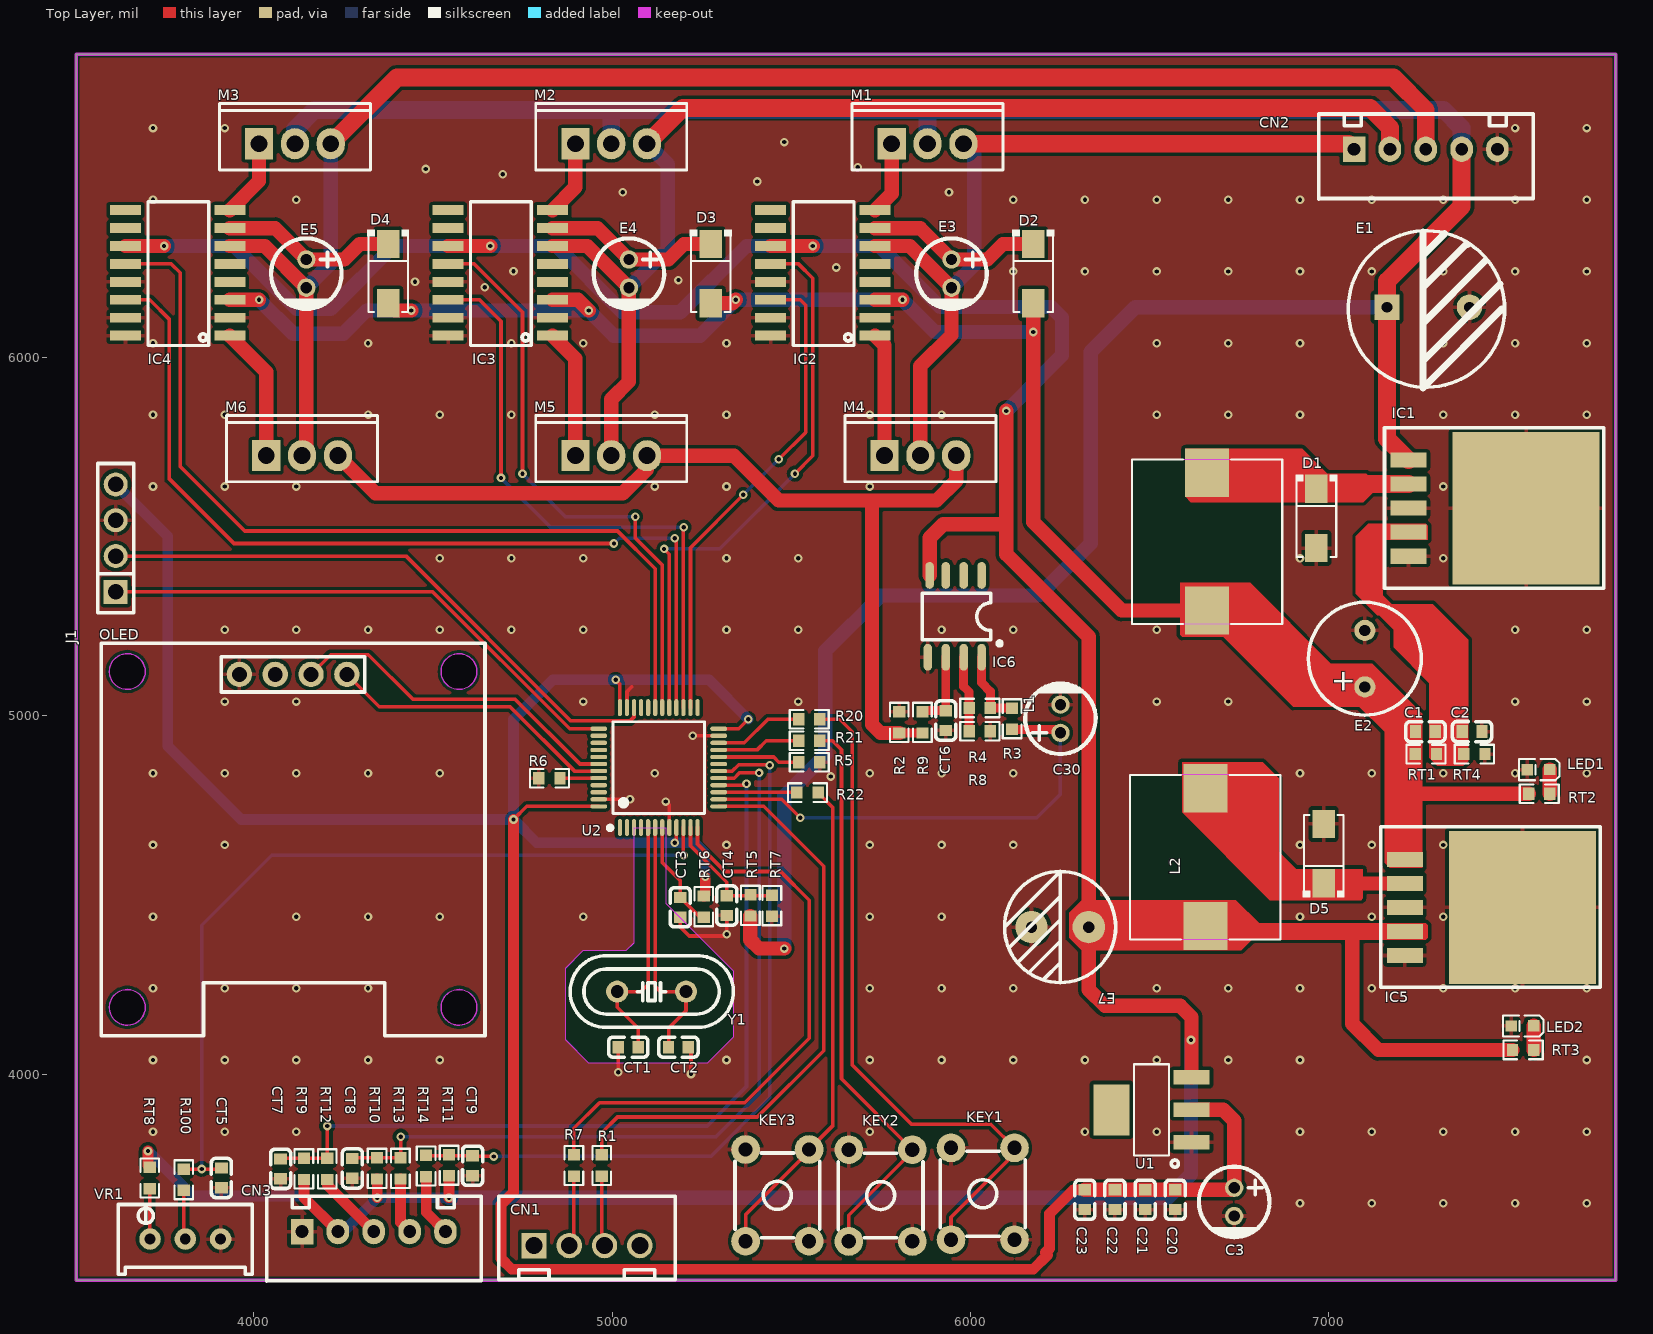
[diagram p0: Top Layer view]
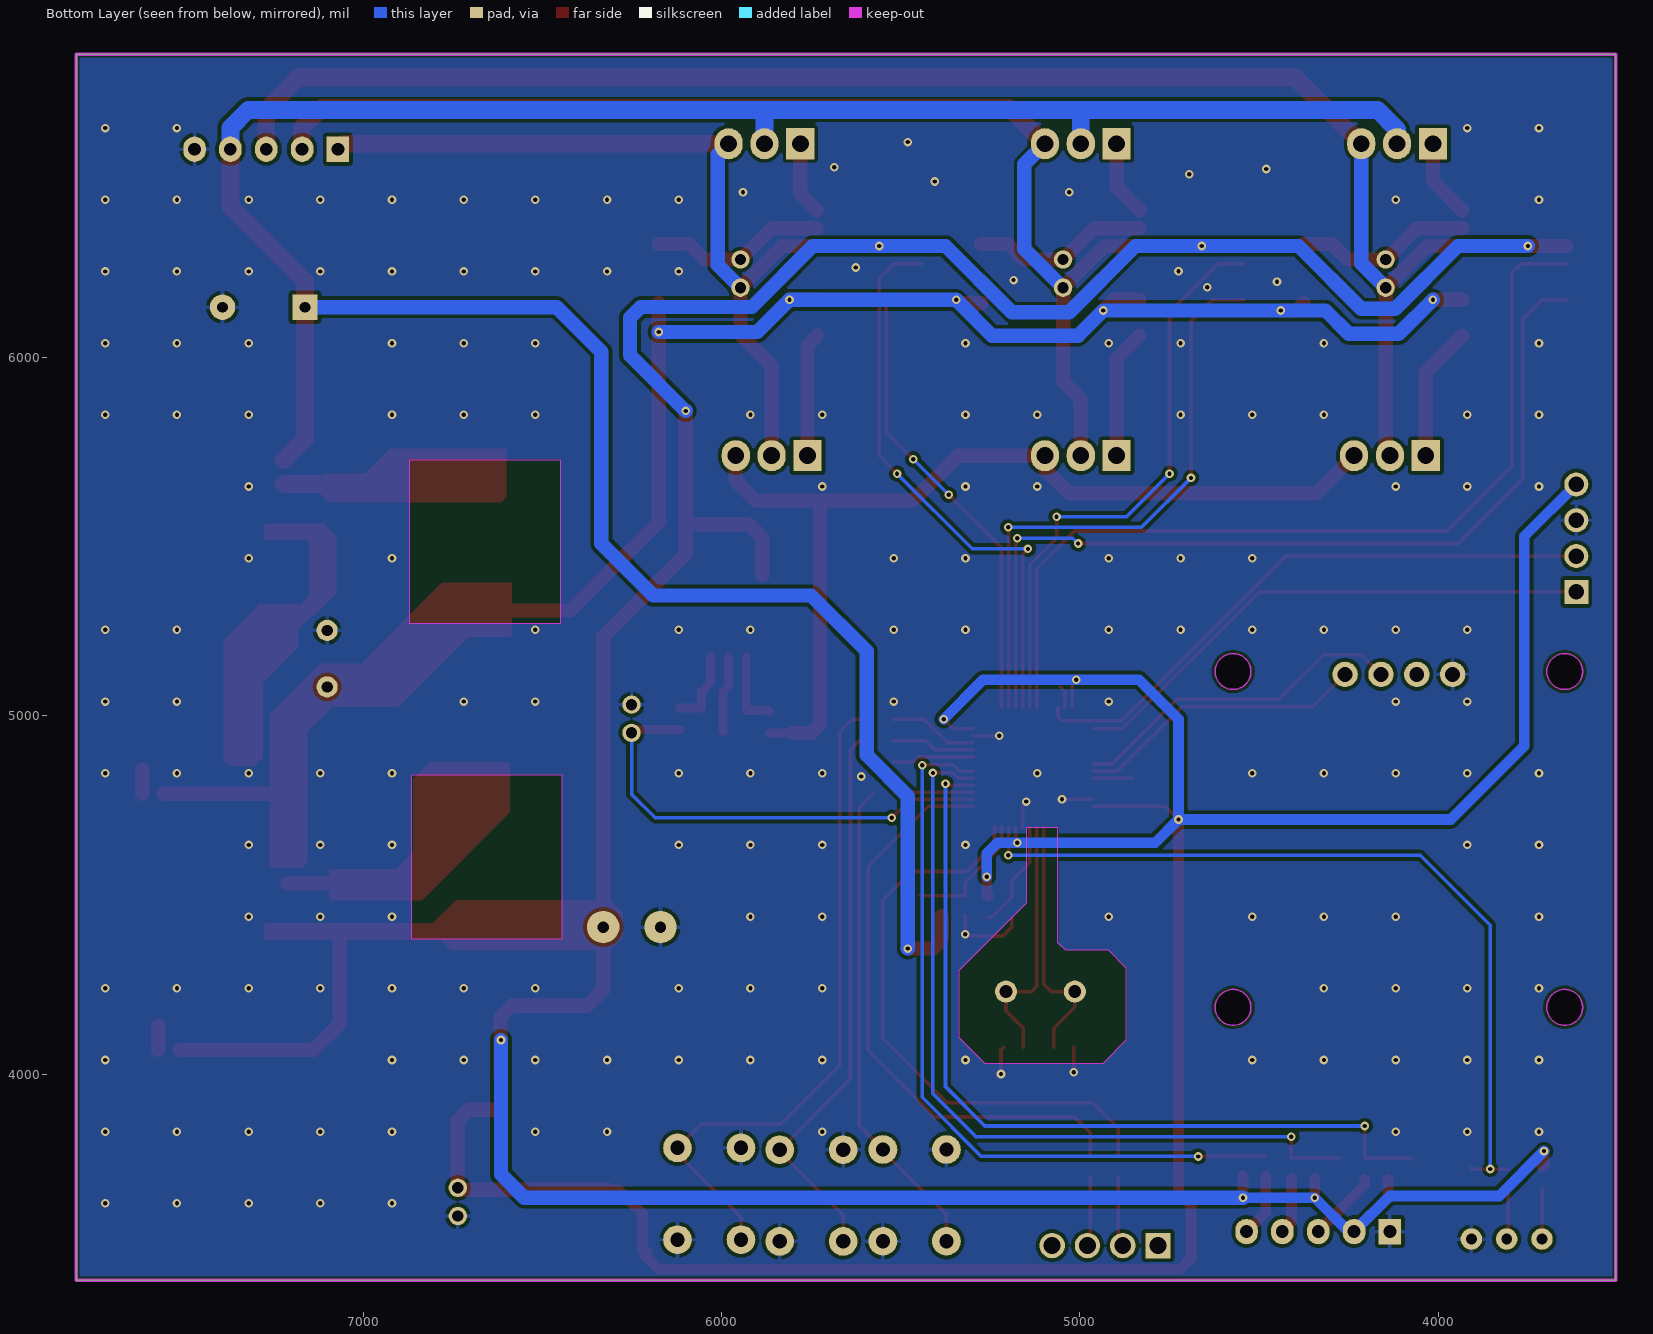
[diagram p1: Bottom Layer view, seen from below]
# Altium PCB MISC58867.pcbdoc
Units mil, origin at the board's own origin, x right, y up, seen from the top; angles counter-clockwise.
Board outline 4295 x 3420 mil, 2 copper layers (Top Layer, Bottom Layer), stack 62.206 mil thick; 83 components, 79 nets, 295 pads, 220 vias.

## Layer stack, top to bottom
Top Solder Mask Layer: solder mask 0.394, Dk 3.3
Top Layer: signal copper 1.379
Dielectric1: surface 59.449, FR4, Dk 4.5
Bottom Layer: signal copper 1.378
Bottom Solder Mask Layer: solder mask 0.394, Dk 3.3

## Board outline
3505,6845 3505,3425 7800,3425 7800,6845

## Design rules (kind name [scope] priority, off if disabled: settings)
BoardOutlineClearance copperThickness2oz_1 [All] p2 off: genericclearance=7.99 ignorepadtopadclearanceinfootprint=FALSE except(0: Arc-SplitContinuation Track-SplitContinuation SMDPad-SplitContinuation THPad-SplitContinuation Via-SplitContinuation Fill-SplitContinuation Region-SplitContinuation Poly-SplitContinuation Text-SplitContinuation Hole-SplitContinuation; 5.98: Arc-CutoutEdge SMDPad-CutoutEdge THPad-CutoutEdge Via-CutoutEdge Fill-CutoutEdge Region-CutoutEdge Text-CutoutEdge; 6.93: Hole-OutlineEdge Hole-CutoutEdge; 10: Poly-OutlineEdge Poly-CutoutEdge; 11.81: Arc-OutlineEdge Track-OutlineEdge SMDPad-OutlineEdge THPad-OutlineEdge Via-OutlineEdge Fill-OutlineEdge Region-OutlineEdge Text-OutlineEdge Track-CutoutEdge)
BoardOutlineClearance copperThickness1oz_1 [All] p4: genericclearance=4.02 ignorepadtopadclearanceinfootprint=FALSE except(0: Arc-SplitContinuation Track-SplitContinuation SMDPad-SplitContinuation THPad-SplitContinuation Via-SplitContinuation Fill-SplitContinuation Region-SplitContinuation Poly-SplitContinuation Text-SplitContinuation Hole-SplitContinuation; 6: SMDPad-CutoutEdge THPad-CutoutEdge Via-CutoutEdge Fill-CutoutEdge Region-CutoutEdge Text-CutoutEdge; 6.93: Hole-OutlineEdge Hole-CutoutEdge; 10: Poly-OutlineEdge Poly-CutoutEdge; 11.8: Arc-OutlineEdge Track-OutlineEdge SMDPad-OutlineEdge THPad-OutlineEdge Via-OutlineEdge Fill-OutlineEdge Region-OutlineEdge Text-OutlineEdge; 11.81: Arc-CutoutEdge Track-CutoutEdge)
Clearance copperThickness2oz [All] p1 off: gap=7.99 ignorepadtopadclearanceinfootprint=FALSE except(5.98: SMDPad-Track SMDPad-SMDPad THPad-Track SMDPad-THPad THPad-THPad Track-Via SMDPad-Via THPad-Via Via-Via Fill-Track Region-Track Fill-SMDPad Region-SMDPad Fill-THPad Region-THPad Fill-Via Region-Via Fill-Fill Fill-Region Region-Region Arc-Track Arc-SMDPad Arc-THPad Arc-Via Fill-Arc Region-Arc Arc-Arc Text-Track SMDPad-Text Text-THPad Text-Via Fill-Text Region-Text Arc-Text Text-Text; 6.93: Hole-Track Hole-SMDPad Hole-THPad Hole-Via Fill-Hole Region-Hole Hole-Arc Hole-Text; 10: Poly-Track Poly-SMDPad Poly-THPad Poly-Via Poly-Fill Poly-Region Poly-Poly Poly-Arc Poly-Text Poly-Hole)
Clearance copperThickness1oz [All] p3: gap=4.02 ignorepadtopadclearanceinfootprint=FALSE except(5.98: SMDPad-Track SMDPad-SMDPad THPad-Track SMDPad-THPad THPad-THPad Track-Via SMDPad-Via THPad-Via Via-Via Fill-Track Region-Track Fill-SMDPad Region-SMDPad Fill-THPad Region-THPad Fill-Via Region-Via Fill-Fill Fill-Region Region-Region; 6: Arc-Track Arc-SMDPad Arc-THPad Arc-Via Fill-Arc Region-Arc Arc-Arc Text-Track SMDPad-Text Text-THPad Text-Via Fill-Text Region-Text Arc-Text Text-Text; 6.93: Hole-Track Hole-SMDPad Hole-THPad Hole-Via Fill-Hole Region-Hole Hole-Arc Hole-Text; 10: Poly-Track Poly-SMDPad Poly-THPad Poly-Via Poly-Fill Poly-Region Poly-Poly Poly-Arc Poly-Text Poly-Hole)
Creepage creepage [All] p1: checkdistance=0 ignoreinternallayers=TRUE applytopolygonpour=TRUE
DiffPairsRouting differentialPair [All] p1: maxlimit=6 minlimit=6 mostfreqgap=6 toplayer_minwidth=5 toplayer_prefwidth=10 toplayer_maxwidth=100 toplayer_mingap=6 toplayer_prefgap=6 toplayer_maxgap=6 bottomlayer_minwidth=5 bottomlayer_prefwidth=10 bottomlayer_maxwidth=100 bottomlayer_mingap=6 bottomlayer_prefgap=6 bottomlayer_maxgap=6 maxuncoupledlength=10
HoleToHoleClearance otherClearance [All] p1: gap=11.81 allowstackedmicrovias=TRUE
Length netLength [All] p1: minlimit=0 maxlimit=0
MatchedLengths netLengthTolerance [All] p1: tolerance=1000
PasteMaskExpansion pasteMaskExpansion [All] p1: expansion=0
PlaneConnect innerPlane [All] p1: planeconnectstyle=Relief reliefexpansion=20 reliefentries=4 reliefconductorwidth=10 reliefairgap=10
PolygonConnect copperRegion [(InNet('GND'))] p1: connectstyle=Relief reliefconductorwidth=10 reliefentries=4 polygonreliefangle="90 Angle" airgapwidth=10 via.connectstyle=Relief via.reliefconductorwidth=10 via.reliefentries=4 via.polygonreliefangle="90 Angle" via.airgapwidth=10
RoutingVias viaSize [All] p1: holewidth=12.01 width=24.02 viastyle="Through Hole" minholewidth=11.81 minwidth=19.68 maxholewidth=248.03 maxwidth=393.7
SolderMaskExpansion solderMaskExpansion [IsVia] p1: expansion=-1000 istentingtop=TRUE
SolderMaskExpansion solderMaskExpansion [All] p2: expansion=2 istentingtop=FALSE
Width copperThickness2oz_2 [All] p1 off: maxlimit=100 minlimit=8 preferedwidth=10
Width copperThickness1oz_2 [All] p2: maxlimit=100 minlimit=5 preferedwidth=10

## Components (designator, comment, footprint, x,y, rotation, side; value= is the part's Value field where it differs from the comment)
C1 "104" C0603 7269.16,4955.29 r0 top
C2 "104" C0603 7399.04,4955.41 r0 top
C3 "16V/220uF" CAP-TH_BD5.0-P2.00-D0.8-FD-10UF50VC110GL 6735.51,3643.15 r270 top
C20 "104" C0603 6571.1,3649.32 r270 top
C21 "104" C0603 6486.97,3649.32 r270 top
C22 "104" C0603 6402.84,3649.32 r270 top
C23 "104" C0603 6318.71,3649.32 r270 top
C30 "106" CAP-TH_BD5.0-P2.00-D0.8-FD-10UF50VC110GL 6250.8,4991.13 r90 top
CN1 "CON4" CON4 4928.57,3546.8 r0 top
CN2 "CON5" CON5 7070,6580 r0 top
CN3 "CON5" CON5 4135.02,3560.37 r0 top
CT1 "30pf" C0603 5045,4075 r180 top
CT2 "30pf" C0603 5185,4075 r180 top
CT3 "105" C0603 5190,4465 r90 top
CT4 "104" C0603 5320,4470 r90 top
CT5 "104" C0603 3910,3710 r90 top
CT6 "104" C0603 5930.8,4986.13 r90 top
CT7 "104" C0603 4075.02,3735.37 r90 top
CT8 "104" C0603 4275.34,3736.44 r90 top
CT9 "104" C0603 4610.63,3744.01 r90 top
D1 "SS34/1N5822" SMA_L4.3-W2.5-LS5.0-RD 6965,5550 r270 top
D2 "M4" SMA_L4.3-W2.5-LS5.0-RD 6175,6232.84 r270 top
D3 "M4" SMA_L4.3-W2.5-LS5.0-RD 5275.07,6232.84 r270 top
D4 "M4" SMA_L4.3-W2.5-LS5.0-RD 4375.14,6232.84 r270 top
D5 "SS34/1N5822" SMA_L4.3-W2.5-LS5.0-RD 6985,4615 r90 top
E1 "50V/330uF" 50v/330uf 7271.97,6134.36 r0 top
E2 "50V/100uF" 50V/100UF 7100,5080 r90 top
E3 "10UF" CAP-TH_BD5.0-P2.00-D0.8-FD-10UF50VC110GL 5946.79,6233.03 r270 top
E4 "10UF" CAP-TH_BD5.0-P2.00-D0.8-FD-10UF50VC110GL 5046.86,6233.03 r270 top
E5 "10UF" CAP-TH_BD5.0-P2.00-D0.8-FD-10UF50VC110GL 4146.93,6233.03 r270 top
E7 "16V/220uF" 16V/220UF 6330,4410 r180 top
IC1 "LM2596S" LM2596S 7385.8,5578.56 r270 top
IC2 "IR2113S" SOP-16 5587.89,6235 r90 top
IC3 "IR2113S" SOP-16 4687.96,6235 r90 top
IC4 "IR2113S" SOP-16 3788.03,6235 r90 top
IC5 "LM2596S-5V" LM2596S 7375.8,4464.72 r270 top
IC6 "LM358" lm358 6030.8,5391.13 r180 top
J1 "CON4(NC)" HDR-TH_4P-P2.54-V-F 3615,5495 r90 top
KEY1 "" SW-PB1 6034.1,3665.9 r270 top
KEY2 "" SW-PB1 5749.1,3660.9 r270 top
KEY3 "" SW-PB1 5460.9,3661.42 r270 top
L1 "33UH/3A" IND-SMD_L11.5-W10.5_MWSA1004 6660,5485 r90 top
L2 "33UH/3A" IND-SMD_L11.5-W10.5_MWSA1004 6655,4605 r90 top
LED1 "REG" LED0603 7584.7,4849.32 r180 top
LED2 "REG" LED0603 7539.7,4134.32 r180 top
M1 "IR540" IR5401 5765,6620.31 r0 top
M2 "IR540" IR5401 4882.5,6620.31 r0 top
M3 "IR540" IR5401 4000,6620.31 r0 top
M4 "IR540" IR5401 5745,5750 r0 top
M5 "IR540" IR5401 4882.5,5750 r0 top
M6 "IR540" IR5401 4020,5750 r0 top
OLED "OLED" OLED 4110,5115 r0 top
R1 "100R" R0603 4970.98,3744.8 r90 top
R2 "0.22R" R0603 5800.8,4981.13 r90 top
R3 "1K" R0603 6115.8,4991.13 r90 top
R4 "10K" R0603 6025.8,5021.13 r0 top
R5 "4.7K" R0603 5550,4870 r180 top
R6 "4.7K" R0603 4825,4825 r0 top
R7 "100R" R0603 4893.28,3744.8 r90 top
R8 "1K" R0603 6025.8,4956.13 r0 top
R9 "1K" R0603 5865.8,4981.13 r90 top
R20 "10K" R0603 5550,4990 r0 top
R21 "10K" R0603 5550,4930 r0 top
R22 "10K" R0603 5545,4785 r0 top
R100 "1K" R0603 3805,3705 r270 top
RT1 "10K" R0603 7270.43,4892.62 r180 top
RT2 "1K" R0603 7586.66,4782 r180 top
RT3 "1K" R0603 7541.66,4067 r180 top
RT4 "1K" R0603 7405.43,4892.62 r180 top
RT5 "20K" R0603 5385.76,4470.48 r270 top
RT6 "10K" R0603 5255.65,4466.9 r90 top
RT7 "1K" R0603 5445.76,4469.52 r90 top
RT8 "5K" R0603 3710,3710 r90 top
RT9 "10K" R0603 4140.02,3735.37 r270 top
RT10 "10K" R0603 4344.26,3736.74 r270 top
RT11 "10K" R0603 4545.02,3745.37 r270 top
RT12 "220R" R0603 4205.02,3735.37 r270 top
RT13 "220R" R0603 4409.26,3736.74 r270 top
RT14 "220R" R0603 4481.13,3743.41 r270 top
U1 "1117-3.3V" 1117-3.3V 6505,3900 r180 top
U2 "STM32F103C8T6" STM32F103C8T6 5130,4855 r90 top
VR1 "10K" R_3296 3809.32,3544.52 r0 top
Y1 "8M" HC-49S_L11.5-W5.0-P4.88 5110,4230 r180 top

## Footprints (in the part's own frame and the unit in brackets; to place one, negate y for a bottom-side part, rotate by r counter-clockwise, add the part's x,y. Pads: shape width x height; smd on the part's side, far side on the other; paste and mask are expansions set on the pad)
16V/220UF [mm]
  round 2.3 hole 0.813 paste+0.051 mask+0.102: 1(0,0) 2(4.064,0)
  silkscreen extent -1.91,-3.94 5.97,3.94
50V/100UF [mm]
  round 1.5 hole 0.8: 1(0,0) 2(4,0)
  silkscreen extent -2,-4 6,4
50v/330uf [mil]
  rect 70.87x70.87 hole 30: 1(-110,5)
  round 70.87 hole 30: 2(120,5)
  silkscreen extent -218,-220 218,218
1117-3.3V [mm]
  rect 2.565x1.015 smd: 1(-2.832,2.3) 2(-2.832,0) 3(-2.832,-2.3)
  rect 2.565x3.6 smd: 4(2.832,0)
  silkscreen extent -1.9,-3.23 1.25,4.06
C0603 [mm]
  rect 0.8x0.9 smd: 1(-0.7,0) 2(0.7,0)
  silkscreen extent -1.39,-0.71 1.39,0.71
CAP-TH_BD5.0-P2.00-D0.8-FD-10UF50VC110GL [mm]
  round 1.3 hole 0.8: 1(-1,0) 2(1,0)
  silkscreen extent -2.5,-2.5 2.5,2.5
CON4 [mm]
  rect 1.8x1.8 hole 1.2: 1(-3.723,-0.648)
  round 1.8 hole 1.2: 2(-1.223,-0.648) 3(1.277,-0.648) 4(3.777,-0.648)
  silkscreen extent -6.22,-3.05 6.28,2.85
CON5 [mm]
  rect 1.6x1.8 hole 0.9: 1(0,0)
  oval 1.6x1.8 hole 0.9: 2(2.54,0) 3(5.08,0) 4(7.62,0) 5(10.16,0)
  silkscreen extent -2.5,-3.52 12.7,2.5
HC-49S_L11.5-W5.0-P4.88 [mm]
  round 1.56 hole 0.9: 1(-2.44,0) 2(2.44,0)
  silkscreen extent -5.8,-2.54 5.77,2.54
HDR-TH_4P-P2.54-V-F [mm]
  rect 1.7x1.7 hole 1.1: 1(-3.81,0)
  round 1.7 hole 1.1: 2(-1.27,0) 3(1.27,0) 4(3.81,0)
  silkscreen extent -5.29,-1.27 5.29,1.27
IND-SMD_L11.5-W10.5_MWSA1004 [mm]
  rect 3.424x3.12 smd: 1(4.878,0) 2(-4.878,0)
  silkscreen extent -5.83,-5.33 5.83,5.33
IR5401 [mm]
  rect 2x2.2 hole 1.2 paste+0 mask+0.102: 1(0.381,-0.635)
  oval 2x2.2 hole 1.2 paste+0 mask+0.102: 2(2.921,-0.635) 3(5.461,-0.635)
  silkscreen extent -2.43,-2.49 8.27,2.22
LED0603 [mm]
  rect 0.8x0.8 smd: 1(-0.799,-0.003) 2(0.799,0.003)
  silkscreen extent -1.49,-0.75 1.39,0.76
lm358 [mm]
  oval 0.6x1.9 smd: 1(0,5.8) 2(1.27,5.8) 3(2.54,5.8) 4(3.81,5.8) 5(0,0) 6(1.27,0) 7(2.54,0) 8(3.683,0)
  silkscreen extent -1.42,1.27 4.19,4.98
LM2596S [mil]
  rect 42x100 smd: 1(-134,-164) 2(-67,-164) 3(0,-164) 4(67,-164) 5(134,-164)
  rect 426x410 smd: 3(0,164)
  silkscreen extent -225,-231 223,381
OLED [mm]
  round 1.8 hole 1.05 paste+0 mask+0.05: 1(-3.81,0) 2(-1.27,0) 3(1.27,0) 4(3.81,0)
  Board Outline Layer circle w0.003: c-11.75,0.2 r1.27
  Board Outline Layer circle w0.003: c11.75,0.2 r1.27
  Board Outline Layer circle w0.003: c11.75,-23.6 r1.27
  Board Outline Layer circle w0.003: c-11.75,-23.6 r1.27
  Board Outline Layer region: -10.48,0.2 -10.606,-0.351 -10.958,-0.793 -11.467,-1.038 -12.033,-1.038 -12.542,-0.793 -12.894,-0.351 -13.02,0.2 -13.02,0.2 -12.894,0.751 -12.542,1.193 -12.033,1.438 -11.467,1.438 -10.958,1.193 -10.606,0.751 -10.48,0.2
  Board Outline Layer region: -10.48,0.2 -10.49,0.041 -10.52,-0.116 -10.569,-0.268 -10.637,-0.412 -10.723,-0.547 -10.824,-0.669 -10.941,-0.779 -11.07,-0.872 -11.209,-0.949 -11.358,-1.008 -11.512,-1.048 -11.67,-1.068 -11.83,-1.068 -11.988,-1.048 -12.142,-1.008 -12.291,-0.949 -12.431,-0.872 -12.56,-0.779 -12.676,-0.669 -12.777,-0.547 -12.863,-0.412 -12.931,-0.268 -12.98,-0.116 -13.01,0.041 -13.02,0.2 -13.01,0.359 -12.98,0.516 -12.931,0.667 -12.863,0.812 -12.777,0.946 -12.676,1.069 -12.56,1.178 -12.431,1.272 -12.291,1.349 -12.142,1.408 -11.988,1.447 -11.83,1.467 -11.67,1.467 -11.512,1.447 -11.358,1.408 -11.209,1.349 -11.07,1.272 -10.941,1.178 -10.824,1.069 -10.723,0.946 -10.637,0.812 -10.569,0.667 -10.52,0.516 -10.49,0.359
  Board Outline Layer region: 13.02,0.2 12.894,-0.351 12.542,-0.793 12.033,-1.038 11.467,-1.038 10.958,-0.793 10.606,-0.351 10.48,0.2 10.48,0.2 10.606,0.751 10.958,1.193 11.467,1.438 12.033,1.438 12.542,1.193 12.894,0.751 13.02,0.2
  Board Outline Layer region: 13.02,0.2 13.01,0.041 12.98,-0.116 12.931,-0.268 12.863,-0.412 12.777,-0.547 12.676,-0.669 12.56,-0.779 12.431,-0.872 12.291,-0.949 12.142,-1.008 11.988,-1.048 11.83,-1.068 11.67,-1.068 11.512,-1.048 11.358,-1.008 11.209,-0.949 11.07,-0.872 10.941,-0.779 10.824,-0.669 10.723,-0.547 10.637,-0.412 10.569,-0.268 10.52,-0.116 10.49,0.041 10.48,0.2 10.49,0.359 10.52,0.516 10.569,0.667 10.637,0.812 10.723,0.946 10.824,1.069 10.941,1.178 11.07,1.272 11.209,1.349 11.358,1.408 11.512,1.447 11.67,1.467 11.83,1.467 11.988,1.447 12.142,1.408 12.291,1.349 12.431,1.272 12.56,1.178 12.676,1.069 12.777,0.946 12.863,0.812 12.931,0.667 12.98,0.516 13.01,0.359
  Board Outline Layer region: 13.02,-23.6 12.894,-24.151 12.542,-24.593 12.033,-24.838 11.467,-24.838 10.958,-24.593 10.606,-24.151 10.48,-23.6 10.48,-23.6 10.606,-23.049 10.958,-22.607 11.467,-22.362 12.033,-22.362 12.542,-22.607 12.894,-23.049 13.02,-23.6
  Board Outline Layer region: 13.02,-23.6 13.01,-23.759 12.98,-23.916 12.931,-24.067 12.863,-24.212 12.777,-24.346 12.676,-24.469 12.56,-24.578 12.431,-24.672 12.291,-24.749 12.142,-24.808 11.988,-24.847 11.83,-24.867 11.67,-24.867 11.512,-24.847 11.358,-24.808 11.209,-24.749 11.07,-24.672 10.941,-24.578 10.824,-24.469 10.723,-24.346 10.637,-24.212 10.569,-24.067 10.52,-23.916 10.49,-23.759 10.48,-23.6 10.49,-23.441 10.52,-23.284 10.569,-23.132 10.637,-22.988 10.723,-22.853 10.824,-22.731 10.941,-22.621 11.07,-22.528 11.209,-22.451 11.358,-22.392 11.512,-22.352 11.67,-22.332 11.83,-22.332 11.988,-22.352 12.142,-22.392 12.291,-22.451 12.431,-22.528 12.56,-22.621 12.676,-22.731 12.777,-22.853 12.863,-22.988 12.931,-23.132 12.98,-23.284 13.01,-23.441
  Board Outline Layer region: -10.48,-23.6 -10.606,-24.151 -10.958,-24.593 -11.467,-24.838 -12.033,-24.838 -12.542,-24.593 -12.894,-24.151 -13.02,-23.6 -13.02,-23.6 -12.894,-23.049 -12.542,-22.607 -12.033,-22.362 -11.467,-22.362 -10.958,-22.607 -10.606,-23.049 -10.48,-23.6
  Board Outline Layer region: -10.48,-23.6 -10.49,-23.759 -10.52,-23.916 -10.569,-24.067 -10.637,-24.212 -10.723,-24.346 -10.824,-24.469 -10.941,-24.578 -11.07,-24.672 -11.209,-24.749 -11.358,-24.808 -11.512,-24.847 -11.67,-24.867 -11.83,-24.867 -11.988,-24.847 -12.142,-24.808 -12.291,-24.749 -12.431,-24.672 -12.56,-24.578 -12.676,-24.469 -12.777,-24.346 -12.863,-24.212 -12.931,-24.067 -12.98,-23.916 -13.01,-23.759 -13.02,-23.6 -13.01,-23.441 -12.98,-23.284 -12.931,-23.132 -12.863,-22.988 -12.777,-22.853 -12.676,-22.731 -12.56,-22.621 -12.431,-22.528 -12.291,-22.451 -12.142,-22.392 -11.988,-22.352 -11.83,-22.332 -11.67,-22.332 -11.512,-22.352 -11.358,-22.392 -11.209,-22.451 -11.07,-22.528 -10.941,-22.621 -10.824,-22.731 -10.723,-22.853 -10.637,-22.988 -10.569,-23.132 -10.52,-23.284 -10.49,-23.441
  Multi-Layer board cut-out: -10.48,0.2 -10.606,-0.351 -10.958,-0.793 -11.467,-1.038 -12.033,-1.038 -12.542,-0.793 -12.894,-0.351 -13.02,0.2 -13.02,0.2 -12.894,0.751 -12.542,1.193 -12.033,1.438 -11.467,1.438 -10.958,1.193 -10.606,0.751 -10.48,0.2
  Multi-Layer board cut-out: 13.02,0.2 12.894,-0.351 12.542,-0.793 12.033,-1.038 11.467,-1.038 10.958,-0.793 10.606,-0.351 10.48,0.2 10.48,0.2 10.606,0.751 10.958,1.193 11.467,1.438 12.033,1.438 12.542,1.193 12.894,0.751 13.02,0.2
  Multi-Layer board cut-out: 13.02,-23.6 12.894,-24.151 12.542,-24.593 12.033,-24.838 11.467,-24.838 10.958,-24.593 10.606,-24.151 10.48,-23.6 10.48,-23.6 10.606,-23.049 10.958,-22.607 11.467,-22.362 12.033,-22.362 12.542,-22.607 12.894,-23.049 13.02,-23.6
  Multi-Layer board cut-out: -10.48,-23.6 -10.606,-24.151 -10.958,-24.593 -11.467,-24.838 -12.033,-24.838 -12.542,-24.593 -12.894,-24.151 -13.02,-23.6 -13.02,-23.6 -12.894,-23.049 -12.542,-22.607 -12.033,-22.362 -11.467,-22.362 -10.958,-22.607 -10.606,-23.049 -10.48,-23.6
  silkscreen extent -13.6,-25.6 13.6,2.2
R0603 [mil]
  rect 31.75x34.02 smd paste-3937.01 mask+2: 1(-29.66,0) 2(29.66,0)
  silkscreen extent -55,-26 55,26
R_3296 [mil]
  round 60 hole 30 paste+0 mask+2: 1(-98.4,-5) 2(0,-5) 3(98.4,-5)
  silkscreen extent -187,-103 187,92
SMA_L4.3-W2.5-LS5.0-RD [mm]
  rect 2x1.593 smd: 1(-2.1,0) 2(2.1,0)
  silkscreen extent -3.11,-1.48 2.73,1.48
SOP-16 [mil]
  rect 27.6x86.6 smd paste+0 mask+4: 1(-175,-145.65) 2(-125,-145.65) 3(-75,-145.65) 4(-25,-145.65) 5(25,-145.65) 6(75,-145.65) 7(125,-145.65) 8(175,-145.65) 9(175,145.65) 10(125,145.65) 11(75,145.65) 12(25,145.65) 13(-25,145.65) 14(-75,145.65) 15(-125,145.65) 16(-175,145.65)
  silkscreen extent -203,-87 199,83
STM32F103C8T6 [mil]
  oval 47.2x11.8 smd paste+0 mask+4: 1(-167.3,108.3) 2(-167.3,88.6) 3(-167.3,68.9) 4(-167.3,49.2) 5(-167.3,29.5) 6(-167.3,9.8) 7(-167.3,-9.8) 8(-167.3,-29.5) 9(-167.3,-49.2) 10(-167.3,-68.9) 11(-167.3,-88.6) 12(-167.3,-108.3) 25(167.3,-108.3) 26(167.3,-88.6) 27(167.3,-68.9) 28(167.3,-49.2) 29(167.3,-29.5) 30(167.3,-9.8) 31(167.3,9.8) 32(167.3,29.5) 33(167.3,49.2) 34(167.3,68.9) 35(167.3,88.6) 36(167.3,108.3)
  oval 11.8x47.2 smd paste+0 mask+4: 13(-108.3,-167.3) 14(-88.6,-167.3) 15(-68.9,-167.3) 16(-49.2,-167.3) 17(-29.5,-167.3) 18(-9.8,-167.3) 19(9.8,-167.3) 20(29.5,-167.3) 21(49.2,-167.3) 22(68.9,-167.3) 23(88.6,-167.3) 24(108.3,-167.3) 37(108.3,167.3) 38(88.6,167.3) 39(68.9,167.3) 40(49.2,167.3) 41(29.5,167.3) 42(9.8,167.3) 43(-9.8,167.3) 44(-29.5,167.3) 45(-49.2,167.3) 46(-68.9,167.3) 47(-88.6,167.3) 48(-108.3,167.3)
  silkscreen extent -174,-128 128,142
SW-PB1 [mil]
  round 80 hole 40 paste+0 mask+2: 1(-127.95,88.58) 2(127.95,-88.58) 3(-127.95,-88.58) 4(127.95,88.58)
  silkscreen extent -118,-118 118,118

## Via types
v1: diameter 24.02, hole 12, Top Layer to Bottom Layer, 220 vias

## Nets (pads, with @x,y where several pads share a name; then routed paths per layer and width w, separated by ;. In a path a pad name is that pad's centre, name@x,y a point inside that pad or via, vN(x,y) a via of type N, cw(c..) or ccw(c..) an arc to the next point about the centre after c; other vN are vias at no path point)
1-HIN: IC2.12 U2.29 | length 1600.7
  Top Layer w10: v1(5145,5465) 5159.5,5450.5 U2.29 ; IC2.12 5520,6260 5560,6220 5560,5725 v1(5510,5675)
  Bottom Layer w10: v1(5145,5465) 5300,5465 v1(5510,5675)
1-LIN: IC2.14 U2.26 | length 1359.8
  Top Layer w10: U2.26 5218.6,5468.6 v1(5365.92,5615.92) ; IC2.14 5525,6160 5540,6145 5540,5790 v1(5465,5715)
  Bottom Layer w10: v1(5365.92,5615.92) v1(5465,5715)
1-VS: CN2.1 E3.2 IC2.6 M1.3 M4.2 | length 2302.7
  Top Layer w40: IC2.6 5830.45,6310 E3.2 5946.79,6061.79 5860,5975 M4.2
  Top Layer w50: M1.3 7054.69,6595.31 CN2.1
  Bottom Layer w40: E3.2 6010,6256.87 6010,6565.31 M1.3
1HO: IC2.8 M1.1 | length 204.6
  Top Layer w40: IC2.8 5780,6456.46 M1.1
1LO: IC2.1 M4.1 | length 346
  Top Layer w40: IC2.1 5760,6033.54 M4.1
2-HIN: IC3.12 U2.30 | length 1642
  Top Layer w10: IC3.12 4615,6260 4750,6125 v1(4750,5675) ; v1(5065,5555) 5065,5495 5139.8,5420.2 U2.30
  Bottom Layer w10: v1(4750,5675) 4870,5555 v1(5065,5555)
2-LIN: IC3.14 U2.27 | length 1679.9
  Top Layer w10: IC3.14 4630,6160 4690,6100 v1(4690,5662.99) ; U2.27 5198.9,5523.9 v1(5200,5525)
  Bottom Layer w10: v1(4690,5662.99) 4827.99,5525 v1(5200,5525)
2-VS: CN2.2 E4.2 IC3.6 M2.3 M5.2 | length 3417.4
  Top Layer w40: IC3.6 4930.52,6310 E4.2 5046.86,5931.86 4997.5,5882.5 M5.2
  Top Layer w50: M2.3 5197.19,6695 7115,6695 7170,6640 CN2.2
  Bottom Layer w40: E4.2 5155,6301.8 5155,6537.81 M2.3
2HO: IC3.8 M2.1 | length 211.8
  Top Layer w40: IC3.8 4897.5,6473.89 M2.1
2LO: IC3.1 M5.1 | length 361.5
  Top Layer w40: IC3.1 4897.5,5996.11 M5.1
3-HIN: IC4.12 U2.31 | length 2533.8
  Top Layer w10: IC4.12 3770,6260 3795,6235 3795,5695 3975,5515 5015,5515 5120.2,5409.8 U2.31
3-LIN: IC4.14 U2.28 | length 2555.6
  Top Layer w10: IC4.14 3710,6160 3765,6105 3765,5660 3945,5480 v1(5005,5480) ; v1(5175,5495) 5179.2,5490.8 U2.28
  Bottom Layer w10: v1(5005,5480) 5020,5495 v1(5175,5495)
3-VS: CN2.3 E5.2 IC4.6 M3.3 M6.2 | length 4443.7
  Top Layer w40: IC4.6 4030.59,6310 E5.2 4146.93,5736.93 M6.2
  Top Layer w50: M3.3 4399.69,6780 7180,6780 7270,6690 CN2.3
  Bottom Layer w40: E5.2 4215,6261.73 M3.3
3HO: IC4.8 M3.1 | length 219
  Top Layer w40: IC4.8 4015,6491.32 M3.1
3LO: IC4.1 M6.1 | length 377
  Top Layer w40: IC4.1 4035,5958.68 M6.1
5V: CN3.2 E7.1 IC2.11 IC3.11 IC4.11 IC5.4 IC6.8 L2.2 RT3.2 RT8.2 RT9.2 RT10.2 RT11.2 U1.3 | length 10605.4
  Top Layer w30: v1(3705,3785) 3705,3744.66 RT8.2 ; RT9.2 4140.02,3655.37 CN3.2 ; RT10.2 4345,3706.34 v1(4345,3655) ; v1(4545,3655) RT11.2
  Top Layer w40: IC4.11 v1(3750,6310) ; IC3.11 v1(4660,6310) ; IC2.11 v1(5559.59,6310) ; IC6.8 5885.8,5495.8 5923.57,5533.57 6100,5533.57 ; v1(6100,5850) 6100,5533.57 ; U1.3 6616.52,4158.48 6585,4190 6375,4190 6330,4235 E7.1 6330,5220 6100,5450 6100,5533.57 ; 7065,4395 7065,4140 7138,4067 RT3.2
  Bottom Layer w30: v1(3705,3785) 3830,3660 4135.39,3660 CN3.2 4250.37,3560.37 v1(4345,3655) v1(4545,3655)
  Bottom Layer w40: v1(3750,6310) 3945,6310 4120,6135 4215,6135 4390,6310 v1(4660,6310) 4845,6310 5030,6125 5190,6125 5375,6310 v1(5559.59,6310) 5745,6310 5915,6140 6225,6140 6255,6110 6255,6005 v1(6100,5850) ; v1(4545,3655) 6550,3655 6615,3720 v1(6615,4095)
13.5V: C1.1 D2.2 D3.2 D4.2 E2.1 IC2.3 IC3.3 IC4.3 IC5.1 L1.2 RT1.2 RT2.2 | length 4282.3
  Top Layer w40: IC4.3 v1(4015,6160) ; D4.2 4395.3,6130 v1(4440,6130) ; IC3.3 4905,6160 v1(4935,6130) ; D3.2 5335.16,6150.16 v1(5345,6160) ; IC2.3 v1(5810,6160) ; D2.2 v1(6175,6070) 6175,5540 6422.05,5292.95 L1.2 ; 7225,4782 RT2.2
  Bottom Layer w40: v1(4015,6160) 4110,6065 4250,6065 4315,6130 v1(4440,6130) v1(4935,6130) 5005,6060 5245,6060 v1(5345,6160) v1(5810,6160) 5900,6070 v1(6175,6070)
24V: CN2.4 E1.1 IC1.1 M1.2 M2.2 M3.2 RT5.2 | length 7893.5
  Top Layer w40: RT5.2 5385.76,4374.24 5410,4350 v1(5480,4350)
  Top Layer w50: IC1.1 7161.97,5772.39 E1.1 7161.97,6211.97 7370,6420 CN2.4
  Bottom Layer w40: v1(5480,4350) 5480,4775 5595,4890 5595,5180 5750,5335 6190,5335 6335,5480 6335,6015 6459.36,6139.36 E1.1
  Bottom Layer w50: M3.2 4115,6635 4170,6690 4998.12,6690 ; M2.2 4997.5,6689.38 4998.12,6690 ; M1.2 5880,6687.56 5877.56,6690 ; CN2.4 7370,6640 7320,6690 5877.56,6690 ; 4998.12,6690 5877.56,6690
$2N3: D1.1 IC1.2 L1.1 | length 262.1
  Top Layer w50: D1.1 6977.88,5645.56 IC1.2
$2N4: C1.2 C2.1 IC1.4 RT1.1 RT4.2
$2N6: D5.1 IC5.2 L2.1 | length 232.2
  Top Layer w40: D5.1@6980,4532.68 6980.96,4531.72 IC5.2
$2N60: R100.2 VR1.2 | length 137.6
  Top Layer w10: R100.2 3805,3543.84 VR1.2
$2N67: CN1.1
$2N89: KEY1.1 KEY1.2 R20.2 | length 1912.5
  Top Layer w10: R20.2 5635,4990 5670,4955 5670,4025 5835,3860 6056.53,3860 KEY1.1 6122.68,3777.68 5945.52,3600.52 KEY1.2@5945.52,3537.95
$2N90: KEY2.1 KEY2.2 R21.2 | length 1598
  Top Layer w10: R21.2 5615,4930 5640,4905 5640,3986.53 KEY2.1 5837.68,3782.68 5660.52,3605.52 KEY2.2@5660.52,3532.95
$2N91: KEY3.1 KEY3.2 R22.2 | length 1368.8
  Top Layer w10: KEY3.2 5372.32,3607.32 5549.48,3784.48 KEY3.1 5615,3854.89 5615,4744.66 R22.2
$2N104: D3.1 E4.1 IC3.7 | length 495.6
  Top Layer w40: IC3.7 4959.26,6360 E4.1 5157.4,6272.4 5200.52,6315.52 D3.1
$2N120: D2.1 E3.1 IC2.7 | length 495.6
  Top Layer w40: IC2.7 5859.19,6360 E3.1 6047.4,6272.4 6090.52,6315.52 D2.1
$2N126: D4.1 E5.1 IC4.7 | length 495.6
  Top Layer w40: IC4.7 4059.33,6360 E5.1 4252.4,6272.4 4295.52,6315.52 D4.1
$2N148: M4.3 M5.3 M6.3 R2.1 R9.1 | length 2754.2
  Top Layer w25: R2.1 R9.1
  Top Layer w40: M6.3 4340,5620 5030,5620 5097.5,5687.5 M5.3 5340,5725 5465,5600 5725.43,5600 ; R2.1 5748.53,4951.47 5725,4975 5725,5599.57 5725.43,5600 ; M4.3 5960,5655 5905,5600 5725.43,5600
$2N158: IC6.1 R3.2 R4.2 | length 212.3
  Top Layer w25: IC6.1 6030.8,5091.54 6055.46,5066.88 R4.2 6115.46,5021.13 R3.2
$2N160: CT6.2 IC6.3 R9.2 | length 215.3
  Top Layer w25: R9.2 5868.7,5013.69 CT6.2 IC6.3
$2N161: IC6.2 R4.1 R8.1 | length 213
  Top Layer w25: IC6.2 5980.8,5081.13 5996.14,5065.79 R4.1 R8.1
$2N178: RT8.1 VR1.1 | length 141.2
  Top Layer w10: RT8.1 3710,3540.44 VR1.1
$2N179: LED1.1 RT2.1 | length 67.5
  Top Layer w40: LED1.1 7616.32,4849.32 RT2.1
$2N180: LED2.1 RT3.1 | length 67.5
  Top Layer w40: LED2.1 7571.32,4134.32 RT3.1
BOOT0: R6.2 U2.44 | length 108.2
  Top Layer w10: R6.2 4855.16,4825.5 U2.44
BOOT1: R5.2 U2.20 | length 229
  Top Layer w10: U2.20 5450.5,4884.5 5465,4870 R5.2
Curr_Adc: C30.1 R3.1 U2.14 | length 1173
  Top Layer w10: U2.14 5473.6,4766.4 v1(5525,4715)
  Bottom Layer w10: v1(5525,4715) 6185,4715 6250.8,4780.8 C30.1
CURR_ADC:  | length 139
  Top Layer w25: 6115.8,4961.47 6241.09,4961.47 6250.8,4951.76
GND: C2.2 C3.2 C20.2 C21.2 C22.2 C23.2 C30.2 CN2.5 CN3.1 CT1.2 CT2.1 CT3.1 CT4.1 CT5.1 CT6.1 CT7.1 CT8.1 CT9.1 D1.2 D5.2 E1.2 E2.2 E7.2 IC1.3 IC1.5 IC2.2 IC2.13 IC2.15 IC2.16 IC3.2 IC3.13 IC3.15 IC3.16 IC4.2 IC4.13 IC4.15 IC4.16 IC5.3 IC5.5 IC6.4 J1.3 KEY1.3 KEY1.4 KEY2.3 KEY2.4 KEY3.3 KEY3.4 LED1.2 LED2.2 OLED.1 R2.2 R5.1 R6.1 R8.2 RT4.1 RT7.1 U1.1 U2.8 U2.23 U2.35 U2.47 VR1.3 | length 669.6
  Top Layer w10: U2.47 v1(5050,4766.4) ; v1(5017.44,4005) CT1.2 ; U2.35 5041.4,5066.4 5055,5080 ; v1(5150,4760) 5159.5,4750.5 U2.8 ; CT3.1 5190,4410 5215,4385 5315,4385 v1(5320,4390) CT4.1 ; CT2.1 5220,4067.56 v1(5220,4000) ; v1(5225,4943.6) U2.23
  other v1: 6919.1,3639.1 7119.1,3639.1 7319.1,3639.1 7519.1,3639.1 7719.1,3639.1 3719.1,3839.1 3919.1,3839.1 4119.1,3839.1 5719.1,3839.1 6319.1,3839.1 6519.1,3839.1 6919.1,3839.1 7119.1,3839.1 7319.1,3839.1 7519.1,3839.1 7719.1,3839.1 3719.1,4039.1 3919.1,4039.1 4119.1,4039.1 4319.1,4039.1 4519.1,4039.1 5319.1,4039.1 5719.1,4039.1 5919.1,4039.1 6119.1,4039.1 6319.1,4039.1 6519.1,4039.1 6719.1,4039.1 6919.1,4039.1 7719.1,4039.1 3719.1,4239.1 3919.1,4239.1 4119.1,4239.1 4319.1,4239.1 5719.1,4239.1 5919.1,4239.1 6119.1,4239.1 6519.1,4239.1 6719.1,4239.1 6919.1,4239.1 7119.1,4239.1 7319.1,4239.1 7519.1,4239.1 7719.1,4239.1 3719.1,4439.1 4119.1,4439.1 4319.1,4439.1 4519.1,4439.1 4919.1,4439.1 5719.1,4439.1 5919.1,4439.1 6919.1,4439.1 7119.1,4439.1 7319.1,4439.1 3719.1,4639.1 3919.1,4639.1 5319.1,4639.1 5719.1,4639.1 5919.1,4639.1 6119.1,4639.1 6919.1,4639.1 7119.1,4639.1 7319.1,4639.1 5610,4830 3719.1,4839.1 3919.1,4839.1 4119.1,4839.1 4319.1,4839.1 4519.1,4839.1 5119.1,4839.1 5719.1,4839.1 5919.1,4839.1 6119.1,4839.1 6919.1,4839.1 7119.1,4839.1 7319.1,4839.1 7519.1,4839.1 7719.1,4839.1 3919.1,5039.1 4119.1,5039.1 4919.1,5039.1 5519.1,5039.1 6519.1,5039.1 6719.1,5039.1 7519.1,5039.1 7719.1,5039.1 3919.1,5239.1 4119.1,5239.1 4319.1,5239.1 4519.1,5239.1 4719.1,5239.1 4919.1,5239.1 5319.1,5239.1 5519.1,5239.1 5919.1,5239.1 6119.1,5239.1 6519.1,5239.1 7519.1,5239.1 7719.1,5239.1 4519.1,5439.1 4719.1,5439.1 4919.1,5439.1 5319.1,5439.1 5519.1,5439.1 6919.1,5439.1 7319.1,5439.1 3719.1,5639.1 3919.1,5639.1 4119.1,5639.1 5119.1,5639.1 5319.1,5639.1 5719.1,5639.1 7319.1,5639.1 3719.1,5839.1 3919.1,5839.1 4319.1,5839.1 4519.1,5839.1 4719.1,5839.1 5119.1,5839.1 5319.1,5839.1 5719.1,5839.1 5919.1,5839.1 6519.1,5839.1 6719.1,5839.1 6919.1,5839.1 7319.1,5839.1 7519.1,5839.1 7719.1,5839.1 3719.1,6039.1 4319.1,6039.1 4719.1,6039.1 4919.1,6039.1 5319.1,6039.1 6519.1,6039.1 6719.1,6039.1 6919.1,6039.1 7319.1,6039.1 7519.1,6039.1 7719.1,6039.1 4645,6195 4450,6210 5185,6215 6119.1,6239.1 6319.1,6239.1 6519.1,6239.1 6719.1,6239.1 6919.1,6239.1 7119.1,6239.1 7319.1,6239.1 7519.1,6239.1 7719.1,6239.1 4725,6240 5625,6250 3719.1,6439.1 4119.1,6439.1 6119.1,6439.1 6319.1,6439.1 6519.1,6439.1 6719.1,6439.1 6919.1,6439.1 7119.1,6439.1 7319.1,6439.1 7519.1,6439.1 7719.1,6439.1 5030,6460 5940,6460 5405,6490 4695,6510 4480,6525 5685,6530 5480,6600 3719.1,6639.1 3919.1,6639.1 7519.1,6639.1 7719.1,6639.1
HALL-A: CN3.3 RT12.2 | length 199.2
  Top Layer w30: RT12.2 4205.02,3690.37 CN3.3
HALL-B: CN3.4 RT13.2 | length 157.4
  Top Layer w30: RT13.2 4409.26,3586.14 CN3.4
HALL-C: CN3.5 RT14.2 | length 175.7
  Top Layer w30: RT14.2 4481.13,3614.26 CN3.5
PA0: CT5.2 R100.1 U2.10 | length 2290.1
  Top Layer w10: R100.1 3907.1,3734.66 CT5.2 ; U2.10 5198.9,4611.1 v1(5200,4610)
  Bottom Layer w10: v1(3855,3735) 3855,4415 4050,4610 v1(5200,4610)
PA1: CT4.2 RT5.1 RT7.2 U2.11 | length 358.6
  Top Layer w10: U2.11 5218.6,4636.4 5320,4535 CT4.2 5444.14,4497.56 RT7.2
PA5: R22.1 U2.15 | length 218.5
  Top Layer w10: U2.15 5514.24,4786.1 R22.1
PA6: CT7.2 RT9.1 RT12.1 U2.16 | length 2360.8
  Top Layer w10: CT7.2 4077.12,3765.03 RT9.1 RT12.1 v1(4205,3855) ; U2.16 5370.8,4805.8 v1(5375,4810)
  Bottom Layer w10: v1(4205,3855) 5265,3855 5375,3965 v1(5375,4810)
PA7: CT8.2 RT10.1 RT13.1 U2.17 | length 2257.2
  Top Layer w10: CT8.2 4277.74,3766.4 RT10.1 RT13.1 4410,3767.15 v1(4410,3825) ; U2.17 5340.5,4825.5 5355,4840 v1(5410,4840)
  Bottom Layer w10: v1(4410,3825) 5290,3825 5410,3945 v1(5410,4840)
PA11: U2.32
PA12: U2.33
PA15: U2.38
PB0: CT9.2 RT11.1 RT14.1 U2.18 | length 2105.1
  Top Layer w10: RT14.1 4482.63,3771.57 CT9.2 4612.2,3770 v1(4670,3770) ; U2.18 5335.2,4845.2 5353.02,4863.02 v1@5440,4863.02
  Bottom Layer w10: v1(4670,3770) 5275,3770 5440,3935 v1(5440,4861.51)
PB1: U2.19
PB3: U2.39
PB4: U2.40
PB5: U2.41
PB6: OLED.3 U2.42 | length 951.9
  Top Layer w10: OLED.3 4215,5170 4320,5170 4445,5045 4730,5045 4910.2,4864.8 U2.42
PB7: OLED.4 U2.43 | length 814.5
  Top Layer w10: OLED.4 4350,5025 4715,5025 4894.8,4845.2 U2.43
PB8: U2.45
PB9: U2.46
PB10: R21.1 U2.21 | length 233.7
  Top Layer w10: U2.21 5404.2,4904.2 5430,4930 R21.1
PB11: R20.1 U2.22 | length 250.4
  Top Layer w10: U2.22 5368.9,4923.9 5435,4990 R20.1
PB12: U2.25
PC13: U2.2
PC14: U2.3
PC15: U2.4
RST: CT3.2 RT6.1 U2.7 | length 304.5
  Top Layer w10: U2.7 5139.8,4590.2 5190,4540 CT3.2 5245.32,4437.24 RT6.1
RXD: R1.2 U2.13 | length 1652.2
  Top Layer w10: R1.2 4970.98,3835.98 5015,3880 5405,3880 5590,4065 5590,4580 5423.3,4746.7 U2.13
RXD1: CN1.3 R1.1 | length 197.1
  Top Layer w10: R1.1 4970.98,3529.16 CN1.3
SWDCLK: J1.1 U2.37 | length 1505.8
  Top Layer w10: J1.1 4500,5345 4881.7,4963.3 U2.37
SWDIO: J1.2 U2.34 | length 1667.4
  Top Layer w10: J1.2 4425,5445 4885,4985 5050,4985 5061.1,4996.1 U2.34
TXD: R7.2 U2.12 | length 1642.4
  Top Layer w10: R7.2 4893.28,3848.28 4965,3920 5370,3920 5550,4100 5550,4485 5470,4565 5315,4565 5238.3,4641.7 U2.12
TXD1: CN1.2 R7.1 | length 199.2
  Top Layer w10: CN1.2 4893.28,3534.15 R7.1
VCC: CN1.4
VCC3.3V: OLED.2
VCC33: C3.1 C20.1 C21.1 C22.1 C23.1 J1.4 RT6.2 U1.2 U2.9 U2.24 U2.36 U2.48 | length 7805.1
  Top Layer w10: v1(4725,4710) 4761.7,4746.7 U2.48 ; v1(5010,5100) 5021.7,5088.3 U2.36 ; v1(5175,4645) 5179.2,4649.2 U2.9 ; U2.24 5353.3,4963.3 v1(5380,4990)
  Top Layer w30: v1(4725,4710) 4725,3670 4690,3635 4690,3485 4720,3455 6175,3455 6215,3495 ; RT6.2 5260,4500.9 v1(5260,4550) ; 6208.23,3501.77 6220,3513.54 6220,3610 6286.88,3676.88 C23.1
  Top Layer w40: C23.1 C22.1 C21.1 C20.1 6729.87,3676.88 C3.1 6735.51,3869.49 6705,3900 U1.2
  Bottom Layer w30: J1.4 3760,5500 3760,4915 3965,4710 v1(4725,4710) ; v1(5260,4550) 5260,4615 5230,4645 v1(5175,4645) 4790,4645 v1(4725,4710) ; v1(5380,4990) 5270,5100 v1(5010,5100) 4835,5100 4725,4990 v1(4725,4710)
Y1: CT1.1 U2.5 Y1.2 | length 711.5
  Top Layer w10: CT1.1 5072.56,4127.44 5013.94,4186.06 Y1.2 5080,4230 5100.5,4250.5 U2.5
Y2: CT2.2 U2.6 Y1.1 | length 710
  Top Layer w10: U2.6 5120.2,4244.8 5135,4230 Y1.1 5206.06,4176.06 5157.44,4127.44 CT2.2
pads on no net: IC2.4 IC2.5 IC2.9 IC2.10 IC3.4 IC3.5 IC3.9 IC3.10 IC4.4 IC4.5 IC4.9 IC4.10 IC6.5 IC6.6 IC6.7 U1.4 U2.1

## Polygon pours and split planes (outlines as drawn)
GND on Top Layer (solid, remove dead copper, pour order 0): 3000,7125 3000,3055 8165,3055 8165,7125
GND on Bottom Layer (solid, remove dead copper, pour order 2): 3195,6945 3195,3000 8090,3000 8090,6945

## Keep-outs
Board Outline Layer:
  region: 6450.31,5714.38 6450.31,5255.62 6869.69,5255.62 6869.69,5714.38
  region: 6445.31,4834.38 6445.31,4375.62 6864.69,4375.62 6864.69,4834.38
  region: 5061.1,4687.7 5149.19,4687.7 5149.19,4475.81 5337.34,4287.66 5337.34,4102.34 5265,4030 4935,4030 4870,4095 4870,4295 4920,4345 5040,4345 5061.1,4366.1
  lines w10: 3505,3425 3505,6845 7800,6845 7800,3425 3505,3425

## Other copper
Top Layer:
  region net $2N3: 6600,5745 6925,5745 6995,5675 7103.75,5675 7122.06,5656.69 7122.06,5622.06 7095,5595 6615,5595 6600,5610
  region net 13.5V: 6585,5370 6780,5370 7005,5145 7120,5145 7260,5005 7260,4575 7170,4575 7155,4590 7155,4955 7085,5025 6900,5025 6705,5220 6590,5220 6585,5225
  region net $2N4: 7270,5535 7275,5530 7275,5490 7155,5490 7150,5485 7150,5335 7175,5310 7290,5310 7388.01,5211.99 7388.01,4873.01 7375,4860 7302.51,4860 7280.2,4882.32 7280.2,5089.8 7180,5190 7180,5240 7140,5280 7135,5280 7075,5340 7075,5500 7110,5535
  region net $2N6: 6590,4870 6815,4870 6860,4825 6860,4620 6908.31,4571.69 7094.73,4571.69 7094.73,4489.73 7090,4485 6835,4485 6590,4730
  region net 5V: 6740,4485 6805,4420 7270,4420 7275,4415 7275,4380 7270,4375 6785,4375 6755,4345 6310,4345 6275,4380 6275,4450 6310,4485